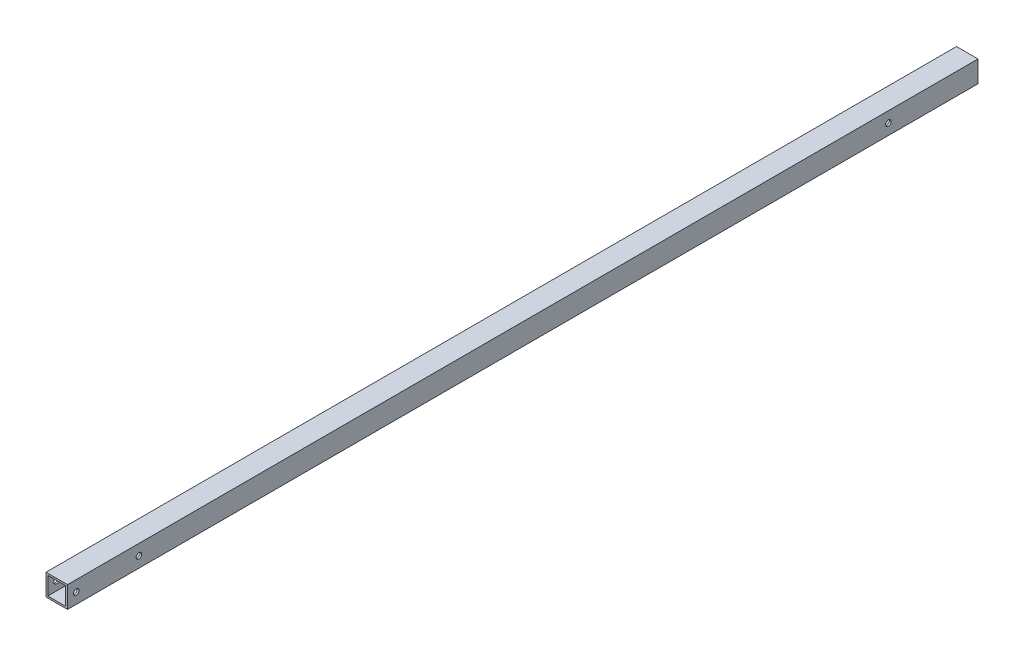
SolidWorks part; units mm, degrees
material "Thornel Mat VMA"
ref_plane "前视基准面" through (0, 0, 0) normal (0, 0, 1) x (1, 0, 0)
ref_plane "上视基准面" through (0, 0, 0) normal (0, 1, 0) x (1, 0, 0)
ref_plane "右视基准面" through (0, 0, 0) normal (1, 0, 0) x (0, 0, -1)
other "Configuration Table"
sketch "草图1" plane through (0, 0, 0) normal (0, 0, 1) x (1, 0, 0)
  line L0 (5, -5) -> (5, 5)
  line L1 (-6, -6) -> (6, -6)
  line L2 (-6, -6) -> (-6, 6)
  line L3 (-6, 6) -> (6, 6)
  line L4 (6, -6) -> (6, 6)
  line L5 (-6, -6) -> (6, 6) construction
  line L6 (-6, 6) -> (6, -6) construction
  line L7 (-5, 5) -> (5, 5)
  line L8 (-5, -5) -> (-5, 5)
  line L9 (-5, -5) -> (5, -5)
  point P0 (0, 0)
  dimension "D1" = 12
  dimension "D2" = 1
extrude "凸台-拉伸1" add sketch "草图1" along normal blind 516
sketch "草图2" plane through (-6, 0, 0) normal (-1, 0, 0) x (0, 0, 1)
  line L0 (0, 6) -> (0, -6) construction
  line L1 (516, 6) -> (0, 6) construction
  line L2 (0, 0) -> (-40.7077, 0) construction
  line L3 (0, 0) -> (284.9629, 284.9629) construction
  line L4 (468.133, 0) -> (234.0665, 234.0665) construction
  circle A0 centre (50, 0) radius 1.55
  circle A1 centre (468.133, 0) radius 1.55
  circle A2 centre (503.133, 0) radius 1.55
  circle A3 centre (75, 0) radius 1.55 construction
  dimension "D1" = 50
  dimension "D2" = 3.1
  dimension "D3" = 6
  dimension "D4" = 35
  dimension "D7" = 25
  dimension "D5" = 135
  dimension "D6" = 331.02
extrude "切除-拉伸1" cut sketch "草图2" against normal through all both and the other way through all
sketch "草图3" plane through (0, 0, 516) normal (0, 0, 1) x (1, 0, 0)
  line L0 (-5, -5) -> (5, -5) construction
  line L1 (5, -5) -> (5, 5) construction
  line L2 (5, 5) -> (-5, 5) construction
  line L3 (-5, 5) -> (-5, -5) construction
  line L4 (6, -6) -> (6, 6)
  line L5 (6, 6) -> (-6, 6)
  line L6 (-6, 6) -> (-6, -6)
  line L7 (-6, -6) -> (6, -6)
  line L8 (6, -6) -> (6, 6)
  line L9 (6, 6) -> (-6, 6)
  line L10 (-6, 6) -> (-6, -6)
  line L11 (-6, -6) -> (6, -6)
  line L12 (-5, -5) -> (5, -5)
  line L13 (5, -5) -> (5, 5)
  line L14 (5, 5) -> (-5, 5)
  line L15 (-5, 5) -> (-5, -5)
  dimension "D1" = 0
extrude "切除-拉伸2" cut sketch "草图3" against normal blind 8
